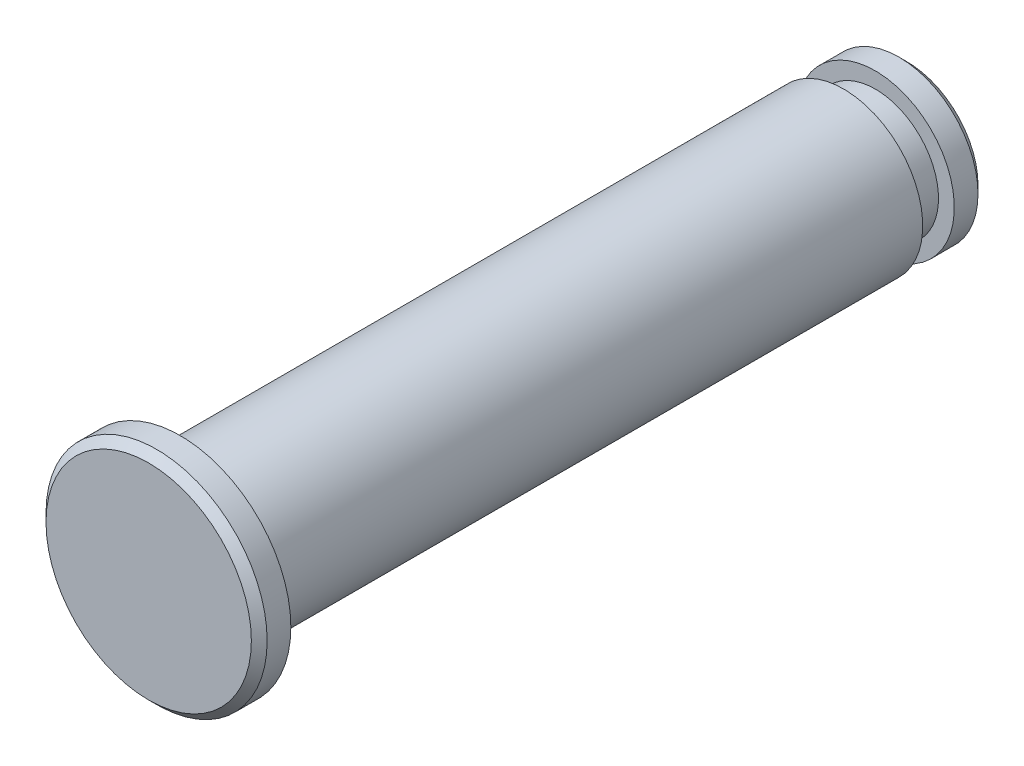
SolidWorks part; units mm, degrees
ref_plane "Front Plane" through (0, 0, 0) normal (0, 0, 1) x (1, 0, 0)
ref_plane "Top Plane" through (0, 0, 0) normal (0, 1, 0) x (1, 0, 0)
ref_plane "Right Plane" through (0, 0, 0) normal (1, 0, 0) x (0, 0, -1)
sketch "Sketch1" plane through (0, 0, 0) normal (0, 0, 1) x (1, 0, 0)
  circle A0 centre (0, 0) radius 5
  dimension "D1" = 10
extrude "Boss-Extrude1" add sketch "Sketch1" along normal blind 46
sketch "Sketch2" plane through (0, 0, 46) normal (0, 0, 1) x (1, 0, 0)
  circle A0 centre (0, 0) radius 7
  dimension "D1" = 14
extrude "Boss-Extrude2" add sketch "Sketch2" along normal blind 2
chamfer "Chamfer1" distance 0.5 angle 45 2 edges at (5, 0, 0) (7, 0, 48)
ref_plane "Plane1" through (0, 0, 2) normal (0, 0, -1) x (-1, 0, 0)
sketch "Sketch3" plane through (0, 0, 2) normal (0, 0, -1) x (-1, 0, 0)
  circle A5 centre (0, 0) radius 5 construction
  circle A6 centre (0, 0) radius 4
  dimension "D1" = 10
  dimension "D2" = 8
extrude "Cut-Extrude-Thin1" cut sketch "Sketch3" against normal blind 2 thin
